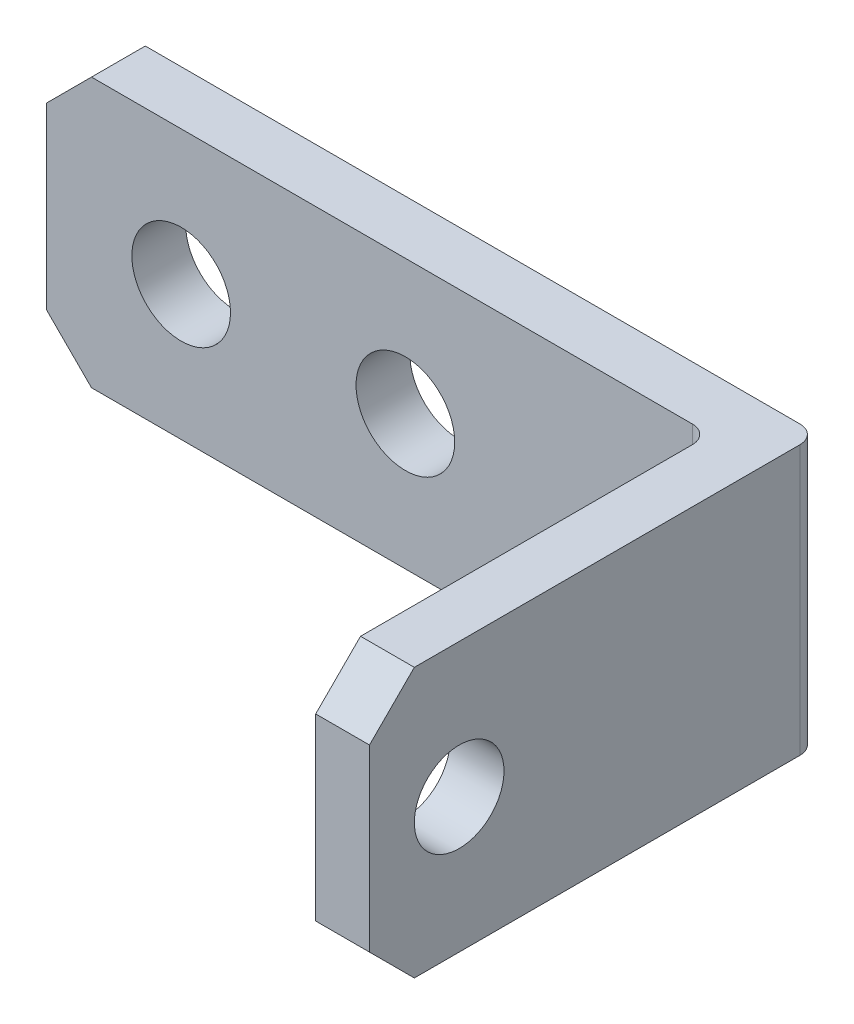
SolidWorks part; units mm, degrees
ref_plane "Front Plane" through (0, 0, 0) normal (0, 0, 1) x (1, 0, 0)
ref_plane "Top Plane" through (0, 0, 0) normal (0, 1, 0) x (1, 0, 0)
ref_plane "Right Plane" through (0, 0, 0) normal (1, 0, 0) x (0, 0, -1)
sketch "Sketch1" plane through (0, 0, 0) normal (0, 0, 1) x (1, 0, 0)
  line L1 (-40, 15) -> (40, 15)
  line L2 (-40, 15) -> (-40, -15)
  line L3 (-40, -15) -> (40, -15)
  line L4 (40, 15) -> (40, -15)
  line L5 (-40, 15) -> (40, -15) construction
  line L6 (-40, -15) -> (40, 15) construction
  circle A0 centre (0, 0) radius 5.5
  circle A1 centre (-25, 0) radius 5.5
  point P0 (0, 0)
  dimension "D4" = 11
  dimension "D1" = 30
  dimension "D2" = 80
  dimension "D3" = 25
extrude "Boss-Extrude1" add sketch "Sketch1" along normal blind 6
sketch "Sketch3" plane through (40, 0, 0) normal (1, 0, 0) x (0, 0, -1)
  line L0 (0, 15) -> (0, -15)
  line L1 (0, 15) -> (-50, 15)
  line L2 (0, -15) -> (-50, -15)
  line L3 (-50, 15) -> (-50, -15)
  circle A0 centre (-40, 0) radius 5
  dimension "D2" = 40
  dimension "D3" = 10
  dimension "D1" = 50
extrude "Boss-Extrude2" add sketch "Sketch3" against normal blind 6
fillet "Fillet1" radius 2 2 edges at (40, 0, 0) (34, 0, 6)
chamfer "Chamfer1" distance 5 angle 45 4 edges at (-40, -15, 3) (-40, 15, 3) (37, 15, 50) (37, -15, 50)
